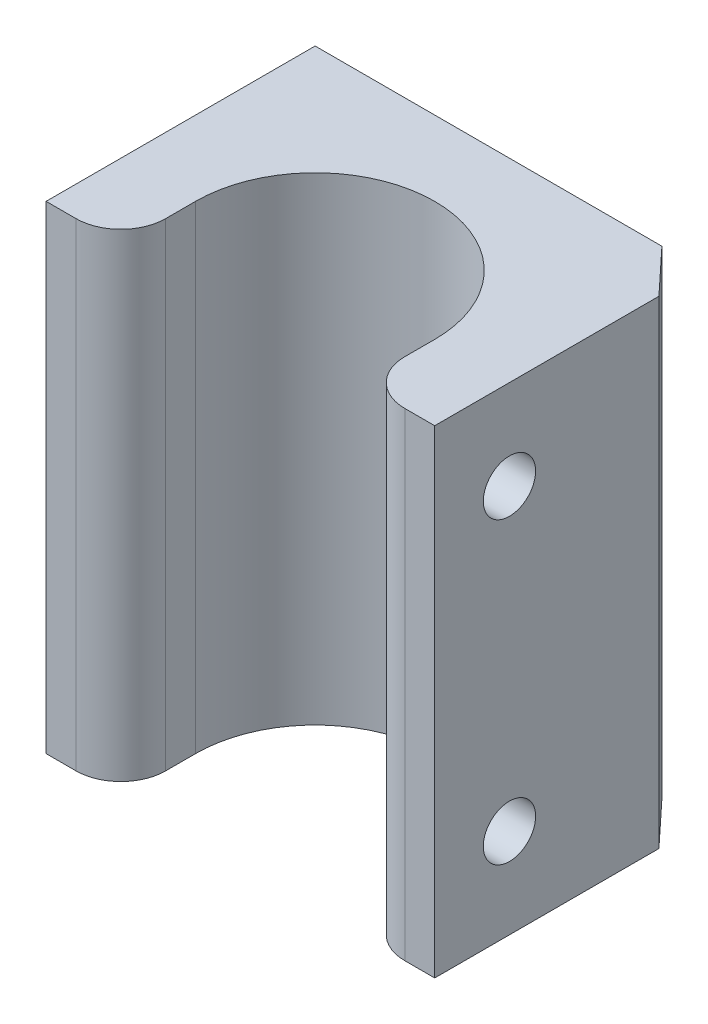
from build123d import *

# Parameters (mm, degrees)
BOSS_EXTRUDE1_DEPTH = 32
SKETCH2_R           = 1.75
CUT_EXTRUDE1_DEPTH  = 10
SKETCH3_W           = 67.397349656
SKETCH3_H           = 25.662976956
CUT_EXTRUDE2_DEPTH  = 38.656340887
SKETCH4_R           = 1.75
CUT_EXTRUDE3_DEPTH  = 10


with BuildPart() as part:
    # Sketch1 → Boss-Extrude1 (new body)
    with BuildSketch(Plane(origin=(0, 0, 0), x_dir=(1, 0, 0), z_dir=(0, 1, 0))):
        with BuildLine():
            Line((-8, -10), (-8, -12))
            ThreePointArc((-8, -12), (-8.878679656, -14.121320344), (-11, -15))
            Line((-11, -15), (-13, -15))
            Line((-13, -15), (-13, 15))
            Line((-13, 15), (-1, 15))
            Line((-1, 15), (13, 0))
            Line((13, 0), (13, -15))
            Line((13, -15), (11, -15))
            ThreePointArc((11, -15), (8.878679656, -14.121320344), (8, -12))
            Line((8, -12), (8, -10))
            ThreePointArc((8, -10), (0, -2), (-8, -10))
        make_face()
    extrude(amount=BOSS_EXTRUDE1_DEPTH)

    # Sketch2 → Cut-Extrude1 (cut)
    with BuildSketch(Plane(origin=(13, 0, 0), x_dir=(0, 0, -1), z_dir=(1, 0, 0))):
        with Locations((-10, 26)):
            Circle(SKETCH2_R)
        with Locations((-10, 6)):
            Circle(SKETCH2_R)
    extrude(amount=-CUT_EXTRUDE1_DEPTH, mode=Mode.SUBTRACT)

    # Sketch3 → Cut-Extrude2 (cut, through all)
    with BuildSketch(Plane(origin=(0, 32, 0), x_dir=(1, 0, 0), z_dir=(0, 1, 0))):
        with Locations((-9.275193266, 15.831488478)):
            Rectangle(SKETCH3_W, SKETCH3_H)
    extrude(amount=-CUT_EXTRUDE2_DEPTH, mode=Mode.SUBTRACT)

    # Sketch4 → Cut-Extrude3 (cut)
    with BuildSketch(Plane.ZY.offset(13)):
        with Locations((0, 6)):
            Circle(SKETCH4_R)
        with Locations((0, 26)):
            Circle(SKETCH4_R)
    extrude(amount=-CUT_EXTRUDE3_DEPTH, mode=Mode.SUBTRACT)


solid = part.part
